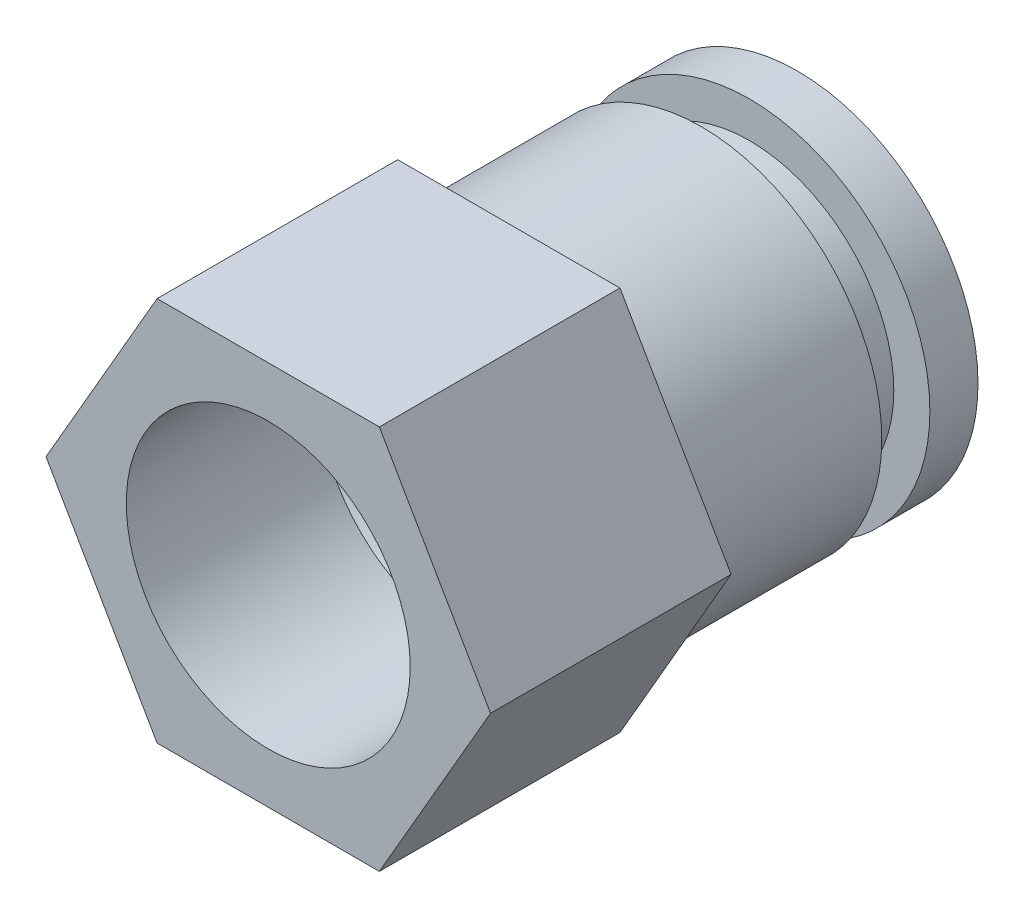
SolidWorks part; units mm, degrees
material "OTHER"
ref_plane "Front Plane" through (0, 0, 0) normal (0, 0, 1) x (1, 0, 0)
ref_plane "Top Plane" through (0, 0, 0) normal (0, 1, 0) x (1, 0, 0)
ref_plane "Right Plane" through (0, 0, 0) normal (1, 0, 0) x (0, 0, -1)
sketch "Sketch1" plane through (0, 0, 0) normal (0, 0, 1) x (1, 0, 0)
  circle A0 centre (0, 0) radius 7.5
  dimension "D1" = 15
extrude "Boss-Extrude1" add sketch "Sketch1" along normal blind 2
sketch "Sketch2" plane through (0, 0, 2) normal (0, 0, 1) x (1, 0, 0)
  circle A0 centre (0, 0) radius 6
  dimension "D1" = 12
extrude "Boss-Extrude2" add sketch "Sketch2" along normal blind 2
sketch "Sketch3" plane through (0, 0, 4) normal (0, 0, 1) x (1, 0, 0)
  circle A0 centre (0, 0) radius 7.5
  dimension "D1" = 15
extrude "Boss-Extrude3" add sketch "Sketch3" along normal blind 8
sketch "Sketch4" plane through (0, 0, 12) normal (0, 0, 1) x (1, 0, 0)
  line L1 (9.2376, 0) -> (4.6188, 8)
  line L2 (4.6188, 8) -> (-4.6188, 8)
  line L3 (-4.6188, 8) -> (-9.2376, 0)
  line L4 (-9.2376, 0) -> (-4.6188, -8)
  line L5 (-4.6188, -8) -> (4.6188, -8)
  line L6 (4.6188, -8) -> (9.2376, 0)
  circle A0 centre (0, 0) radius 8 construction
  dimension "D1" = 16
extrude "Boss-Extrude4" add sketch "Sketch4" along normal blind 10
sketch "Sketch5" plane through (0, 0, 0) normal (0, 0, -1) x (-1, 0, 0)
  circle A0 centre (0, 0) radius 3
  dimension "D1" = 6
extrude "Cut-Extrude1" cut sketch "Sketch5" against normal through all
hole_wizard "G1/4 Tapped Hole1" positions "Sketch6" profile "Sketch7" tap size "G1/4" standard "ISO"
sketch "Sketch6" plane through (0, 0, 22) normal (0, 0, 1) x (1, 0, 0)
  point P0 (0, 0)
cosmetic thread "Cosmetic thread1"
sketch "Sketch7" plane through (0, 0, 22) normal (1, 0, 0) x (0, -1, 0)
  line L0 (0, 0) -> (0, 11.5451)
  line L1 (0, 11.5451) -> (5.9, 8)
  line L2 (5.9, 8) -> (5.9, 0)
  line L5 (5.9, 0) -> (0, 0)
  line L10 (0, 11.5451) -> (-5.9, 8) construction
  line L11 (0, -6.35) -> (0, 107.95) construction
  dimension "螺纹孔钻头直径" = 11.8
  dimension "螺纹孔钻头深度" = 8
  dimension "导头角度" = 118
